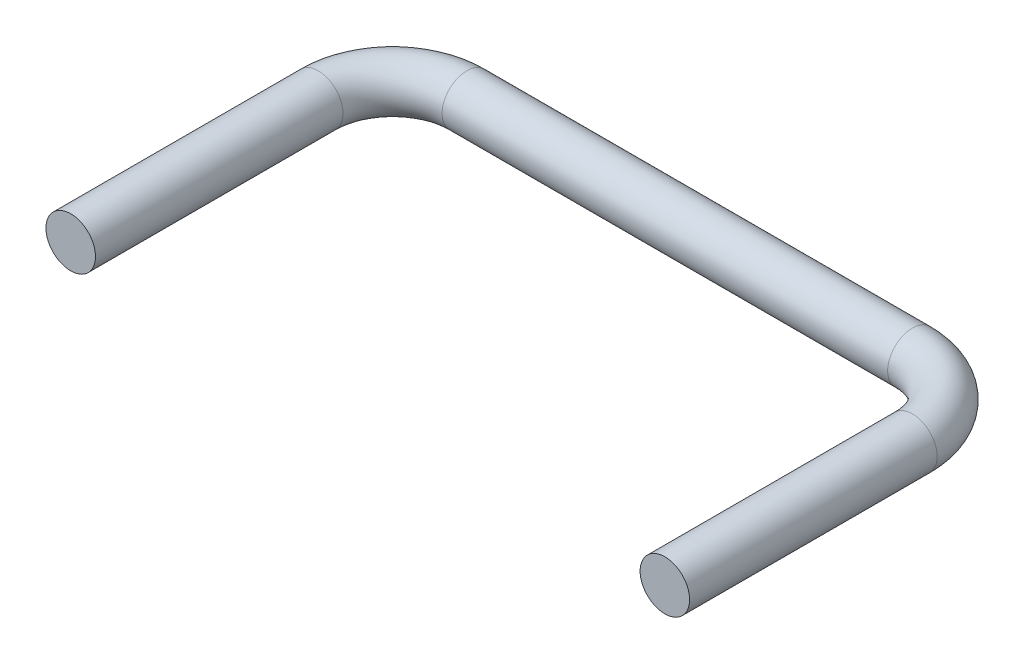
from build123d import *

# Parameters (mm, degrees)
SKETCH1_R = 6.35


with BuildPart() as part:
    # Sweep1: sweep along a path in Sketch2
    with BuildLine(Plane(origin=(0, 0, 0), x_dir=(1, 0, 0), z_dir=(0, 1, 0))) as sweep1_path:
        Line((0, 0), (0, 63.5))
        ThreePointArc((0, 63.5), (5.579615818, 76.970384182), (19.05, 82.55))
        Line((19.05, 82.55), (133.35, 82.55))
        ThreePointArc((133.35, 82.55), (146.820384182, 76.970384182), (152.4, 63.5))
        Line((152.4, 63.5), (152.4, 0))
    # Sketch1 → Sweep1 (sweep)
    with BuildSketch(Plane.XY):
        Circle(SKETCH1_R)
    sweep(path=sweep1_path.line)


solid = part.part
